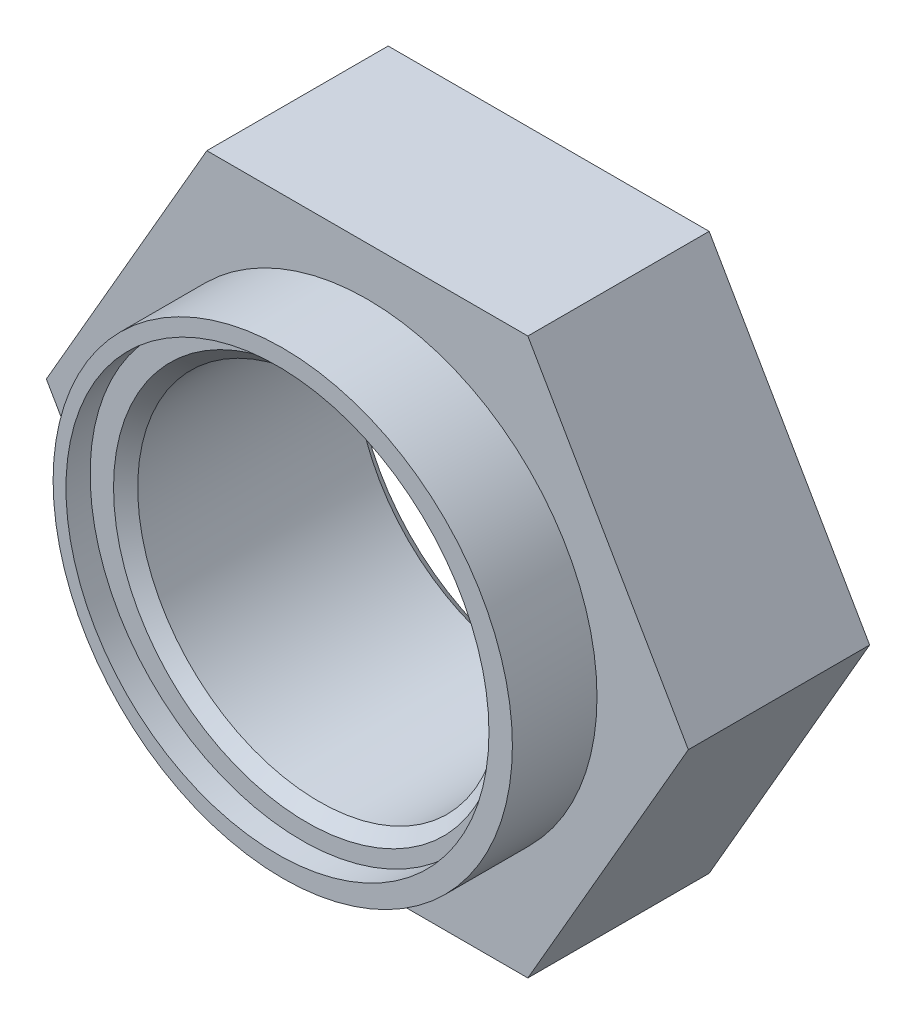
from build123d import *

# Parameters (mm, degrees)
SKETCH_1_R          = 19
EXTRUDE_1_DEPTH     = 7
EXTRUDE_2_DEPTH     = 15
SKETCH_3_R          = 17.5
CUT_EXTRUDE_1_DEPTH = 2
SKETCH_4_R          = 15
CUT_EXTRUDE_2_DEPTH = 41.426888742
CHAMFER_1_SIZE      = 1


with BuildPart() as part:
    # 草图1 → 凸台-拉伸1 (new body)
    with BuildSketch(Plane.XY):
        Circle(SKETCH_1_R)
    extrude(amount=-EXTRUDE_1_DEPTH)

    # 草图2 → 凸台-拉伸2 (add)
    with BuildSketch(Plane(origin=(0, 0, -7), x_dir=(-1, 0, 0), z_dir=(0, 0, -1))):
        Polygon((13.279056191, -23), (26.558112383, 0), (13.279056191, 23), (-13.279056191, 23), (-26.558112383, 0), (-13.279056191, -23), align=None)
    extrude(amount=EXTRUDE_2_DEPTH)

    # 草图3 → 切除-拉伸1 (cut)
    with BuildSketch(Plane.XY):
        with Locations((-0.437352874, 0)):
            Circle(SKETCH_3_R)
    extrude(amount=-CUT_EXTRUDE_1_DEPTH, mode=Mode.SUBTRACT)

    # 草图4 → 切除-拉伸2 (cut, through all)
    with BuildSketch(Plane.XY.offset(-2)):
        Circle(SKETCH_4_R)
    extrude(amount=-CUT_EXTRUDE_2_DEPTH, mode=Mode.SUBTRACT)

    # 倒角1
    chamfer_1_edges = [part.edges().sort_by_distance(p)[0] for p in [
        (-15, 0, -22),
        (-15, 0, -2),
    ]]
    chamfer(chamfer_1_edges, length=CHAMFER_1_SIZE)


solid = part.part
